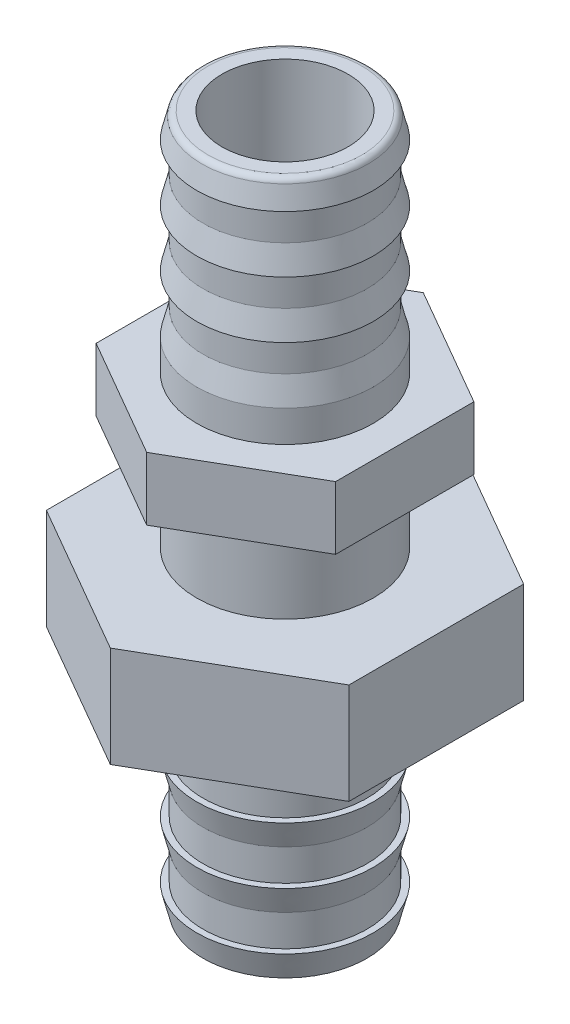
SolidWorks part; units mm, degrees
material "AISI 304"
ref_plane "Front Plane" through (0, 0, 0) normal (0, 0, 1) x (1, 0, 0)
ref_plane "Top Plane" through (0, 0, 0) normal (0, 1, 0) x (1, 0, 0)
ref_plane "Right Plane" through (0, 0, 0) normal (1, 0, 0) x (0, 0, -1)
sketch "Sketch2" plane through (0, 0, 0) normal (0, 1, 0) x (1, 0, 0)
  circle A0 centre (0, 0) radius 7
  dimension "D1" = 14
extrude "Boss-Extrude1" add sketch "Sketch2" along normal blind 18
sketch "Sketch5" plane through (0, 0, 0) normal (0, -1, 0) x (1, 0, 0)
  line L1 (9.5, -5.4848) -> (9.5, 5.4848)
  line L2 (9.5, 5.4848) -> (0, 10.9697)
  line L3 (0, 10.9697) -> (-9.5, 5.4848)
  line L4 (-9.5, 5.4848) -> (-9.5, -5.4848)
  line L5 (-9.5, -5.4848) -> (0, -10.9697)
  line L6 (0, -10.9697) -> (9.5, -5.4848)
  circle A0 centre (0, 0) radius 9.5 construction
  dimension "D1" = 19
extrude "Boss-Extrude2" add sketch "Sketch5" along normal blind 5
sketch "Sketch6" plane through (0, -5, 0) normal (0, -1, 0) x (1, 0, 0)
  circle A1 centre (0, 0) radius 7
  circle A2 centre (0, 0) radius 7
  dimension "D1" = 0
extrude "Boss-Extrude3" add sketch "Sketch6" along normal blind 32
sketch "Sketch4" plane through (0, 18, 0) normal (0, 1, 0) x (1, 0, 0)
  circle A0 centre (0, 0) radius 5
  dimension "D1" = 10
extrude "Cut-Extrude1" cut sketch "Sketch4" against normal through all
sketch "Sketch3" plane through (0, 0, 0) normal (0, 0, 1) x (1, 0, 0)
  line L0 (0, 0) -> (0, 64.2773) construction
  line L1 (6.5, 18) -> (7, 16)
  line L2 (7, 16) -> (6.5, 16)
  line L7 (7, 18) -> (-7, 18) construction
  line L8 (7, 0) -> (7, 18) construction
  line L9 (6.5, 18) -> (7, 18)
  line L10 (7, 18) -> (7, 2.5)
  line L11 (-7, 9) -> (14.6266, 9) construction
  line L12 (-7, 18) -> (-7, 0) construction
  line L13 (6.5, 16) -> (6.5, 13.5)
  line L14 (6.5, 13.5) -> (7, 11.5)
  line L15 (7, 11.5) -> (6.5, 11.5)
  line L16 (6.5, 11.5) -> (6.5, 9)
  line L17 (6.5, 9) -> (7, 7)
  line L18 (7, 7) -> (6.5, 7)
  line L20 (6.5, 7) -> (6.5, 4.5)
  line L21 (6.5, 4.5) -> (7, 2.5)
  line L22 (-7, 18) -> (-7, -37) construction
  line L23 (-7, -9.5) -> (-21.4592, -9.5) construction
  line L24 (-7, -28) -> (14.6266, -28) construction
  line L25 (6.5, -23.5) -> (7, -21.5)
  line L26 (6.5, -26) -> (6.5, -23.5)
  line L27 (7, -26) -> (6.5, -26)
  line L28 (6.5, -28) -> (7, -26)
  line L29 (6.5, -30.5) -> (6.5, -28)
  line L30 (7, -30.5) -> (6.5, -30.5)
  line L31 (6.5, -32.5) -> (7, -30.5)
  line L32 (6.5, -35) -> (6.5, -32.5)
  line L33 (7, -37) -> (7, -21.5)
  line L34 (6.5, -37) -> (7, -37)
  line L35 (7, -35) -> (6.5, -35)
  line L36 (6.5, -37) -> (7, -35)
  dimension "D1" = 6.5
  dimension "D2" = 2
  dimension "D3" = 4.5
  dimension "D4" = 0.5
revolve "Cut-Revolve1" cut sketch "Sketch3" angle 360 about L0
fillet "Fillet1" radius 0.5 1 edges at (0, 18, -6.5)
ref_plane "Plane1" through (0, -12, 0) normal (0, -1, 0) x (-1, 0, 0)
sketch "Sketch8" plane through (0, -12, 0) normal (0, -1, 0) x (-1, 0, 0)
  line L1 (0, 13.8564) -> (-12, 6.9282)
  line L2 (-12, 6.9282) -> (-12, -6.9282)
  line L3 (-12, -6.9282) -> (0, -13.8564)
  line L4 (0, -13.8564) -> (12, -6.9282)
  line L5 (12, -6.9282) -> (12, 6.9282)
  line L6 (12, 6.9282) -> (0, 13.8564)
  circle A0 centre (0, 0) radius 12 construction
  circle A1 centre (0, 0) radius 7 construction
  circle A2 centre (0, 0) radius 7
  dimension "D1" = 24
extrude "Boss-Extrude4" add sketch "Sketch8" along normal blind 8 separate body
